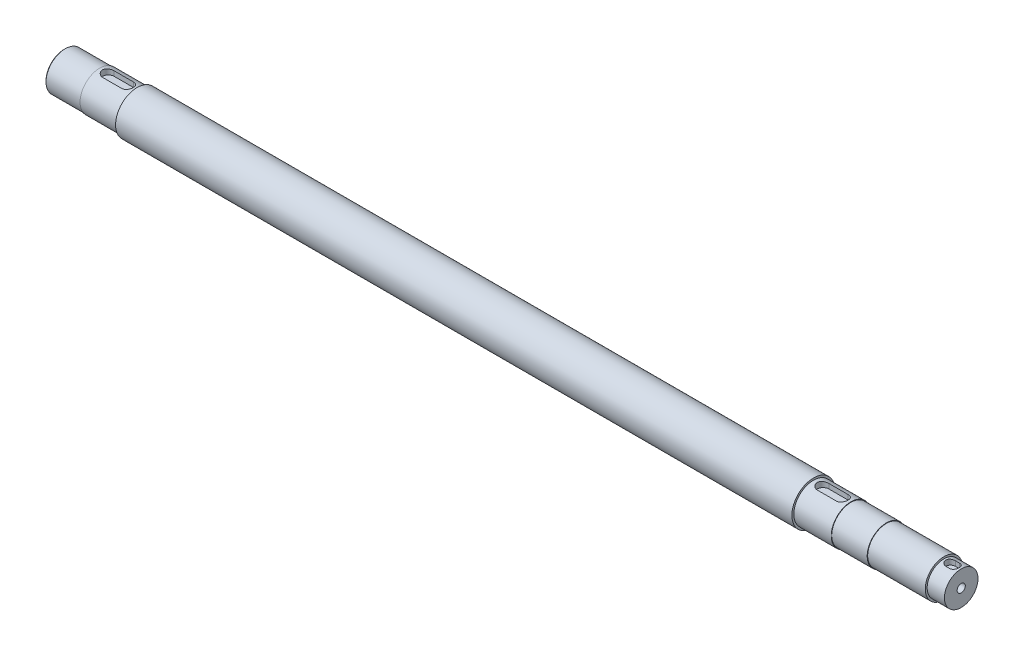
SolidWorks part; units mm, degrees
ref_plane "前视基准面" through (0, 0, 0) normal (0, 0, 1) x (1, 0, 0)
ref_plane "上视基准面" through (0, 0, 0) normal (0, 1, 0) x (1, 0, 0)
ref_plane "右视基准面" through (0, 0, 0) normal (1, 0, 0) x (0, 0, -1)
sketch "草图1" plane through (0, 0, 0) normal (1, 0, 0) x (0, 0, -1)
  circle A0 centre (0, 0) radius 22.5
extrude "凸台-拉伸1" add sketch "草图1" along normal blind 705
sketch "草图2" plane through (705, 0, 0) normal (1, 0, 0) x (0, 0, -1)
  circle A0 centre (0, 0) radius 20.5
extrude "凸台-拉伸2" add sketch "草图2" along normal blind 39
sketch "草图3" plane through (744, 0, 0) normal (1, 0, 0) x (0, 0, -1)
  circle A0 centre (0, 0) radius 20
extrude "凸台-拉伸3" add sketch "草图3" along normal blind 37
sketch "草图4" plane through (781, 0, 0) normal (1, 0, 0) x (0, 0, -1)
  circle A0 centre (0, 0) radius 19.5
extrude "凸台-拉伸4" add sketch "草图4" along normal blind 60
sketch "草图5" plane through (841, 0, 0) normal (1, 0, 0) x (0, 0, -1)
  circle A0 centre (0, 0) radius 17.5
extrude "凸台-拉伸5" add sketch "草图5" along normal blind 18
sketch "草图6" plane through (0, 0, 0) normal (-1, 0, 0) x (0, 0, 1)
  circle A0 centre (0, 0) radius 20.5
extrude "凸台-拉伸6" add sketch "草图6" along normal blind 39
sketch "草图7" plane through (-39, 0, 0) normal (-1, 0, 0) x (0, 0, 1)
  circle A0 centre (0, 0) radius 20
extrude "凸台-拉伸7" add sketch "草图7" along normal blind 37
chamfer "倒角1" distance 1 angle 45 1 edges at (-76, 0, 20)
ref_plane "基准面1" through (0, 20.5, 0) normal (0, 1, 0) x (1, 0, 0)
sketch "草图8" plane through (0, 20.5, 0) normal (0, 1, 0) x (1, 0, 0)
  line L0 (-10, 0) -> (-30, 0) construction
  line L1 (-10, -6) -> (-30, -6)
  line L2 (-10, 6) -> (-30, 6)
  line L3 (0, 22.5) -> (0, -22.5) construction
  line L4 (715, 0) -> (735, 0) construction
  line L5 (715, 6) -> (735, 6)
  line L6 (715, -6) -> (735, -6)
  line L7 (705, -22.5) -> (705, 22.5) construction
  arc A0 (-10, -6) -> (-10, 6) centre (-10, 0) ccw
  arc A1 (-30, 6) -> (-30, -6) centre (-30, 0) ccw
  arc A2 (715, 6) -> (715, -6) centre (715, 0) ccw
  arc A3 (735, -6) -> (735, 6) centre (735, 0) ccw
  point P3 (-20, 0)
  point P12 (725, 0)
  dimension "D1" = 20
  dimension "D2" = 6
  dimension "D3" = 10
  dimension "D4" = 20
  dimension "D5" = 6
  dimension "D6" = 10
extrude "切除-拉伸1" cut sketch "草图8" against normal blind 5.9
ref_plane "基准面2" through (0, 17.5, 0) normal (0, 1, 0) x (1, 0, 0)
sketch "草图9" plane through (0, 17.5, 0) normal (0, 1, 0) x (1, 0, 0)
  line L0 (848, 0) -> (852, 0) construction
  line L1 (848, 5) -> (852, 5)
  line L2 (848, -5) -> (852, -5)
  line L3 (841, -19.5) -> (841, 19.5) construction
  arc A0 (848, 5) -> (848, -5) centre (848, 0) ccw
  arc A1 (852, -5) -> (852, 5) centre (852, 0) ccw
  point P3 (850, 0)
  dimension "D1" = 4
  dimension "D2" = 5
  dimension "D3" = 7
extrude "切除-拉伸2" cut sketch "草图9" against normal blind 5.73
hole_wizard "M10 螺纹孔1" positions "草图11" profile "草图10" tap size "M10" standard "Iso"
sketch "草图11" plane through (859, 0, 0) normal (1, 0, 0) x (0, 0, -1)
  point P0 (0, 0)
sketch "草图10" plane through (859, 0, 0) normal (0, 1, 0) x (0, 0, -1)
  line L0 (0, 0) -> (0, 17.5537)
  line L1 (0, 17.5537) -> (4.25, 15)
  line L2 (4.25, 15) -> (4.25, 0)
  line L5 (4.25, 0) -> (0, 0)
  line L10 (0, 17.5537) -> (-4.25, 15) construction
  line L11 (0, -6.35) -> (0, 107.95) construction
  dimension "螺纹孔钻头直径" = 8.5
  dimension "螺纹孔钻头深度" = 15
  dimension "导头角度" = 118
cosmetic thread "孔螺蚊线1" parameters "D1"=15, "D2"=10
